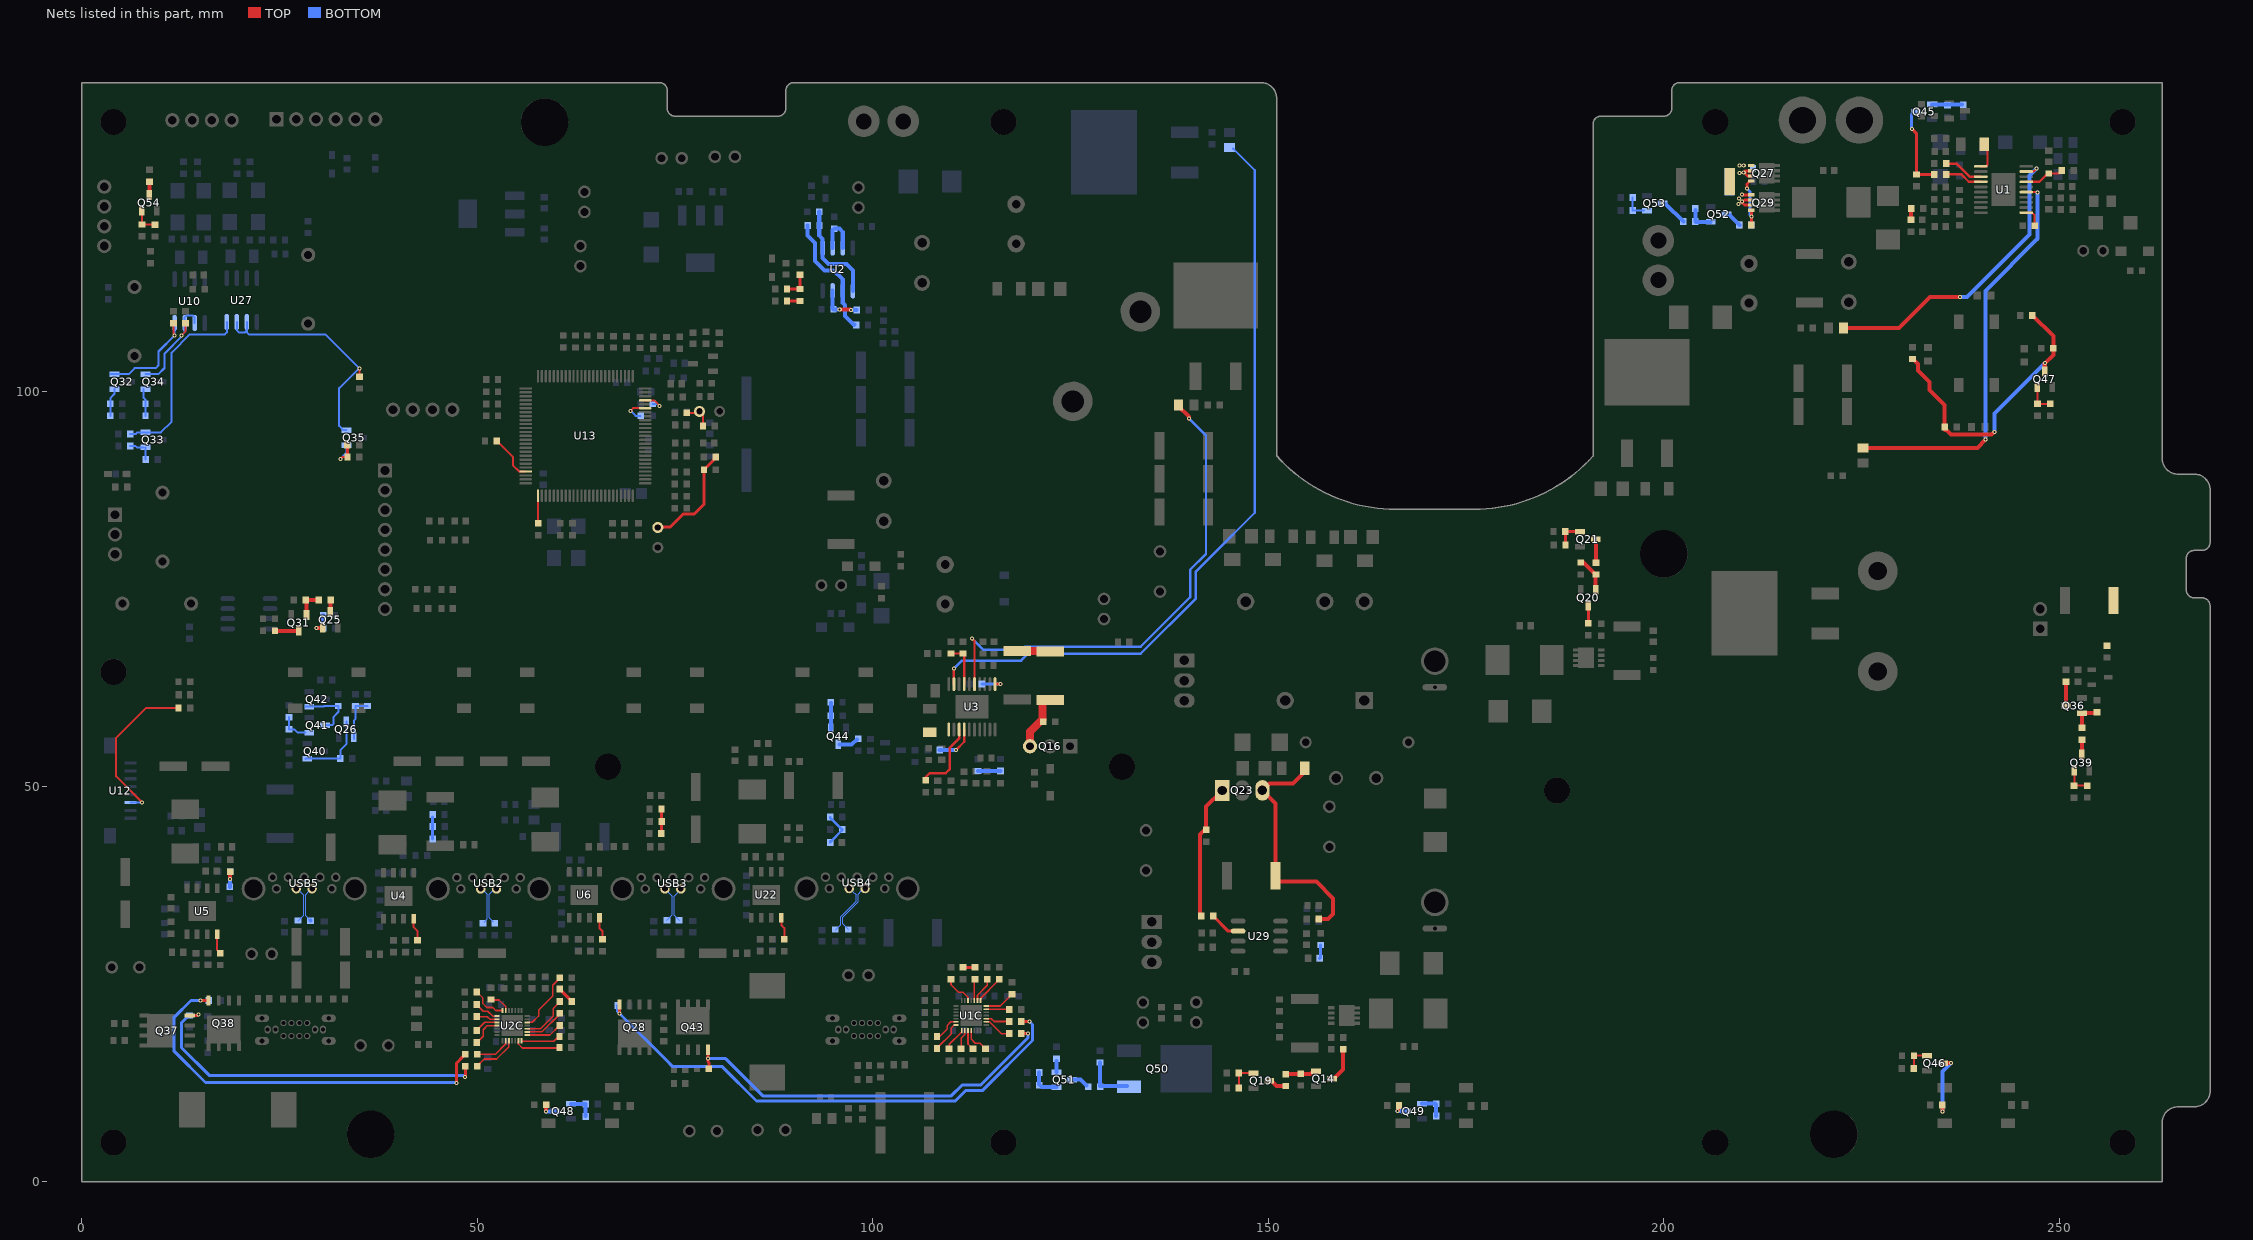
[diagram p0: the nets of this part, all layers, seen from the top]
# Altium PCB MISC84402.PcbDoc (part 8 of 12)
Units mm, origin at the board's own origin, x right, y up, seen from the top; angles counter-clockwise.
Board outline 269.06 x 139 mm, 4 copper layers (TOP, GND02, PWR03, BOTTOM), stack 0.732 mm thick; 694 components, 428 nets, 1859 pads, 1384 vias.

## Via types
v1: diameter 0.508, hole 0.254, TOP to BOTTOM, tented both sides, 1015 vias
v2: diameter 0.508, hole 0.254, TOP to BOTTOM, 243 vias
v3: diameter 0.508, hole 0.305, TOP to BOTTOM, 60 vias
v4: diameter 0.61, hole 0.305, TOP to BOTTOM, 55 vias
v5: diameter 0.61, hole 0.305, TOP to BOTTOM, tented both sides, 8 vias
v6: diameter 0.762, hole 0.381, TOP to BOTTOM, 2 vias
v7: diameter 0.762, hole 0.381, TOP to BOTTOM, tented both sides, 1 vias

## Nets (pads, with @x,y where several pads share a name; then routed paths per layer and width w, separated by ;. In a path a pad name is that pad's centre, name@x,y a point inside that pad or via, vN(x,y) a via of type N, cw(c..) or ccw(c..) an arc to the next point about the centre after c; other vN are vias at no path point) (continued)
NetQ14_1: Q14.1 R23.2 R29.1 | length 3.5
  TOP w0.508: R29.1@152.232,13.673 155.329,13.673 Q14.1@155.626,13.97
NetQ14_3: Q14.3 R61.1 | length 4.1
  TOP w0.508: Q14.3@158.032,13.047 158.233,13.047 159.436,14.249 R61.1@159.436,16.459
NetQ16_3: Q16.3 R50.1 R148.1 | length 5.5
  TOP w1.016: Q16.3@119.888,55.499 119.888,56.947 121.437,58.496 R50.1@121.437,60.342
NetQ19_1: Q19.1 R32.2 R65.1 | length 3.6
  TOP w0.254: R32.2@146.184,13.76 Q19.1@148.114,13.76 ; R65.1@146.294,11.887 R32.2@146.294,13.528
NetQ19_3: Q19.3 R29.2 | length 2.2
  TOP w0.508: Q19.3@150.114,12.81 150.334,12.81 151.003,12.141 R29.2@152.044,12.141
NETQ20_1: Q20.1 R35.2 R39.1 | length 4.2
  TOP w0.508: R35.2@189.789,78.384 191.385,76.788 Q20.1@191.385,74.879
NetQ20_3: Q20.3 R66.1 | length 2
  TOP w0.381: R66.1@190.444,70.619 Q20.3@190.444,72.599
NetQ21_1: Q21.1 R40.2 R44.1 | length 3.3
  TOP w0.381: R40.2@187.554,80.645 187.554,82.079 187.687,82.213 Q21.1@189.389,82.213
NetQ21_3: Q21.3 R39.2 | length 2.8
  TOP w0.508: R39.2@191.415,78.366 Q21.3@191.415,81.127
NETQ23_1: Q23.1 R240.2 R265.2 | length 17.4
  TOP w0.508: R240.2@141.63,33.706 141.326,34.01 141.326,43.917 R265.2@141.942,44.533 ; Q23.1@144.171,49.495 142.139,47.463 R265.2@142.139,44.533 ; R265.2@141.942,44.533 R265.2@142.139,44.533 ; R265.2@141.942,44.533 R265.2@142.139,44.533
NETQ23_3: Q23.3 R258.1 R316.2 R361.1 | length 31.1
  TOP w0.508: R361.1@154.432,51.689 153.111,50.368 150.114,50.368 Q23.3@149.251,49.505 150.902,47.854 150.902,43.272 R316.2@150.902,38.7 150.902,37.549 151.326,37.973 156.066,37.973 158.174,35.865 158.174,33.884 157.529,33.239 R258.1@156.354,33.239
NetQ25_1: Q25.1 R186.2 R193.1 | length 3.2
  TOP w0.508: v2(29.676,70.062) 29.686,70.053 Q25.1@30.455,70.053
  BOTTOM w0.508: v2(29.676,70.062) 30.489,70.062 R193.1@30.489,71.644
NetQ25_3: Q25.3 R100.1 | length 1.6
  TOP w0.508: Q25.3@31.41,72.069 R100.1@31.41,73.625
NETQ26_1: Q26.1 R95.2 R140.2 | length 5.8
  BOTTOM w0.254: Q26.1@34.377,55.992 Q26.1@34.377,56.242 34.377,58.319 34.57,58.512 R140.2@34.57,60.171 R95.2@36.094,60.171
NETQ26_3: Q26.3 Q40.1 R144.1 | length 9.5
  BOTTOM w0.254: Q40.1@28.24,53.498 28.301,53.559 28.49,53.559 R144.1@32.674,53.559 32.674,54.602 33.427,55.355 Q26.3@33.427,58.242
NETQ27_1: Q27.1 Q27.2 Q27.3 Q29.1 Q29.2 Q29.3 R26.2 R45.2 R67.1 | length 6
  TOP w0.381: v1(209.866,124.851) 209.907,124.81 Q29.1@211.06,124.81 ; v1(210.101,127.645) v1@210.12,127.645 ; Q29.3@211.06,123.51 210.191,123.51 209.866,123.835 210.191,124.16 Q29.2@211.06,124.16 ; Q27.3@211.06,127.193 210.572,127.193 v1@210.12,127.645 ; Q27.2@211.06,127.843 210.318,127.843 v1@210.12,127.645
  other v1: 209.892,123.937 210.101,128.534
  other v2: 209.448,123.647 209.499,124.358 209.575,127.584 209.575,128.524
NETQ27_4: Q27.4 Q29.4 R56.2 R60.2 | length 7.6
  TOP w0.381: v1(210.501,125.613) 210.501,126.162 210.882,126.543 Q27.4@211.06,126.543 ; Q29.4@211.06,122.699 Q29.4@211.06,122.86 ; R56.2@211.065,120.98 Q29.4@211.065,122.699
  BOTTOM w0.381: v1(210.501,125.613) 210.882,125.232 210.882,122.264 ; R60.2@211.055,120.99 v1@211.055,121.977
  other v1: 211.087,122.06
NETQ28_4: Q28.4 R126.1 R129.2 | length 66.1
  TOP w0.381: v1(67.971,21.301) Q28.4@67.971,22.431 ; R129.2@118.745,20.285 v1(119.787,20.285)
  BOTTOM w0.381: R126.1@67.726,22.317 67.726,21.546 v1(67.971,21.301) 73.897,15.375 ; 74.087,15.185 73.897,15.375 ; v1(119.787,20.285) v1@119.82,20.252 ; v1@119.837,20.269 120.193,19.914 120.193,17.882 113.894,11.582 111.76,11.582 110.429,10.252 85.278,10.252 80.899,14.63 74.641,14.63 73.897,15.375
NetQ31_1: Q31.1 R98.2 R100.2 | length 3.3
  TOP w0.508: Q31.1@28.39,71.697 R98.2@28.39,73.526 ; R98.2@28.473,73.558 R100.2@29.955,73.558
NetQ31_3: Q31.3 R42.1 | length 3
  TOP w0.508: R42.1@24.401,69.688 Q31.3@27.442,69.688
NETQ32_1: Q32.1 R91.2 R159.2 | length 3.6
  BOTTOM w0.254: R159.2@3.599,96.866 3.582,96.883 3.582,98.39 3.582,99.111 4.096,99.626 Q32.1@4.096,100.234
NETQ32_2: Q32.2 R154.1 U10.4 | length 14.3
  TOP w0.254: R154.1@11.583,108.567 11.583,107.28 11.71,107.153 v1(11.71,107.026)
  BOTTOM w0.254: Q32.2@3.614,102.134 Q32.2@4.096,102.134 5.911,102.134 6.664,102.887 9.331,102.887 9.678,103.234 9.678,104.994 v1(11.71,107.026) U10.4@11.71,108.603
NETQ33_1: Q33.1 R105.2 R165.2 | length 3.3
  BOTTOM w0.254: R105.2@6.104,93.073 R105.2@6.122,93.056 6.757,93.056 6.945,92.868 Q33.1@7.793,92.868 ; Q33.1@8.043,92.868 8.043,91.348 R165.2@8.061,91.33
NETQ33_2: Q33.2 R152.1 U27.4 | length 24
  BOTTOM w0.254: R152.1@6.104,94.58 6.811,94.58 6.999,94.768 Q33.2@8.043,94.768 9.975,94.768 11.329,96.122 11.329,104.858 13.624,107.153 18.06,107.153 18.314,107.407 U27.4@18.314,108.73
NETQ34_1: Q34.1 R93.2 R184.2 | length 3.5
  BOTTOM w0.254: Q34.1@7.809,100.234 7.809,99.124 8.036,98.898 R93.2@8.036,98.39 R184.2@8.036,96.866
NETQ34_2: Q34.2 R156.1 U10.2 U10.3 | length 14.1
  TOP w0.254: v1(12.599,107.026) 13.107,107.534 R156.1@13.107,108.567
  BOTTOM w0.254: Q34.2@8.059,102.134 9.667,102.134 10.44,102.907 10.44,104.74 12.599,106.899 v1(12.599,107.026) 12.98,107.407 U10.3@12.98,108.603 12.98,109.312 13.234,109.566 13.996,109.566 14.25,109.312 U10.2@14.25,108.603
NETQ35_1: Q35.1 R146.2 R176.2 | length 4.6
  TOP w0.254: v1(32.67,91.41) 32.919,91.659 R176.2@33.571,91.659
  TOP w0.381: R146.2@33.554,93.183 33.554,91.676 R176.2@33.571,91.659
  BOTTOM w0.254: v1(32.67,91.41) 33.433,92.173 Q35.1@33.433,93.157
NETQ35_2: Q35.2 R157.1 U27.2 U27.3 | length 30.6
  TOP w0.254: R157.1@35.078,101.819 v1(35.078,102.835)
  BOTTOM w0.254: U27.3@19.584,108.73 19.584,107.661 19.838,107.407 20.6,107.407 20.854,107.661 ; U27.2@20.854,108.73 20.854,107.661 ; Q35.2@33.433,95.057 33.061,95.057 32.512,95.606 32.512,100.355 v1@34.976,102.819 ; v1@35.019,102.776 v1(35.078,102.835) ; v1@35.047,102.865 v1(35.078,102.835) ; v1@35.052,102.87 30.769,107.153 21.108,107.153 20.854,107.407 20.854,107.661 ; v1@35.078,102.962 v1(35.078,102.835)
NetQ36_1: Q36.1 R288.2 R289.2 | length 3.5
  TOP w0.508: R288.2@252.85,57.487 Q36.1@252.85,59.29 R289.2@254.552,59.29
NetQ36_3: Q36.3 R71.1 | length 2.7
  TOP w0.508: Q36.3@250.85,60.24 R71.1@250.85,62.966
NETQ37_4: Q37.4 R201.2 R212.1 | length 45.6
  TOP w0.381: Q37.4@13.615,21.047 14.631,21.047 v1(14.758,21.174) ; v1(48.447,13.301) 48.464,13.319 R201.2@48.464,14.622
  BOTTOM w0.381: v1(14.758,21.174) 14.631,21.046 13.503,21.046 12.599,20.143 12.599,16.983 16.145,13.437 48.31,13.437 v1@48.447,13.3
NETQ38_4: Q38.4 R202.2 R209.1 | length 51.9
  TOP w0.381: v1(15.012,22.952) 15.025,22.939 Q38.4@16.028,22.939 ; v1(47.355,12.539) 47.355,15.021 R202.2@48.285,15.951 ; R202.2@48.285,16.146 R202.2@48.456,16.146
  BOTTOM w0.381: R209.1@16.037,22.952 v1(15.012,22.952) 13.782,22.952 11.659,20.828 11.659,16.526 15.612,12.573 47.319,12.573 v1@47.355,12.538
NetQ39_1: Q39.1 R272.1 R287.2 | length 3.3
  TOP w0.254: Q39.1@251.899,52.026 251.899,50.158 251.943,50.114 R272.1@253.289,50.114
NetQ39_3: Q39.3 R288.1 | length 1.7
  TOP w0.508: Q39.3@252.849,54.026 R288.1@252.849,55.736
NETQ41_1: Q41.1 R180.2 R188.1 | length 3.8
  BOTTOM w0.254: R180.2@26.188,58.774 R188.1@26.188,57.233 26.832,57.233 27.265,56.8 Q41.1@28.24,56.8
NETQ41_3: Q41.3 Q42.1 R319.1 | length 7.8
  BOTTOM w0.254: Q42.1@28.24,60.102 Q42.1@28.74,60.102 30.563,60.102 30.633,60.172 R319.1@32.411,60.171 32.411,59.419 31.81,58.818 31.81,57.929 31.631,57.75 Q41.3@30.74,57.75
NETQ43_4: Q43.4 R130.2 R131.1 | length 49.3
  TOP w0.381: Q43.4@79.147,16.728 v1(79.147,15.586) 79.147,15.205 79.265,15.087 R131.1@79.265,14.316 ; R130.2@118.745,18.761 v1(119.596,18.761)
  BOTTOM w0.381: v1(79.147,15.586) 81.392,15.586 86.091,10.887 109.896,10.887 111.252,12.243 113.614,12.243 119.583,18.212 v1@119.583,18.644 ; v1@119.596,18.644 v1(119.596,18.761)
NetQ44_1: Q44.1 R53.1 R73.2 | length 3.3
  BOTTOM w0.508: Q44.1@94.698,57.27 R73.2@94.698,60.535
NetQ44_3: Q44.3 R104.1 | length 2.5
  BOTTOM w0.508: Q44.3@95.775,55.287 97.324,55.287 R104.1@97.993,55.956
NetQ45_1: Q45.1 R308.2 R314.2 | length 3.8
  BOTTOM w0.508: Q45.1@233.902,136.239 R308.2@237.712,136.239
NetQ45_3: Q45.3 R52.1 R296.2 | length 10.4
  TOP w0.381: v2(231.394,133.121) 231.927,132.588 R296.2@231.927,127.372 ; R296.2@232.181,127.381 R52.1@234.197,127.381
  BOTTOM w0.381: v2(231.394,133.121) 231.292,133.223 231.292,134.925 Q45.3@231.673,135.306
NetQ46_1: Q46.1 R323.1 R325.2 | length 3.1
  TOP w0.254: R325.2@231.622,14.452 R323.1@231.622,15.96 Q46.1@233.232,15.96
NetQ46_3: Q46.3 R64.2 | length 9
  TOP w0.508: v2(235.204,8.915) R64.2@235.204,9.601 ; Q46.3@235.28,15.02 v2(236.313,15.02)
  BOTTOM w0.508: v2(235.204,8.915) 235.204,11.049 ; 235.204,10.279 235.204,11.049 ; v2@236.22,14.961 235.204,13.945 235.204,11.049
NetQ47_1: Q47.1 R332.1 R333.2 | length 3.8
  TOP w0.254: Q47.1@247.244,100.533 247.244,98.382 247.244,98.374 R332.1@248.86,98.374
NetQ47_3: Q47.3 R78.2 R79.2 R118.2 R187.2 | length 37.5
  TOP w0.508: R79.2@231.521,104.038 232.156,103.403 232.156,102.616 233.604,101.168 233.604,100.136 235.509,98.231 R118.2@235.509,95.453 ; R118.2@235.458,95.326 R118.2@235.518,95.267 ; R118.2@235.518,95.063 R118.2@235.518,95.267 ; R118.2@235.518,95.453 R118.2@235.518,95.267 ; v2@241.783,94.818 241.452,94.488 236.296,94.488 R118.2@235.518,95.267 ; R187.2@246.558,109.626 249.25,106.934 249.25,104.572 248.158,103.48 Q47.3@248.158,102.565 ; Q47.3@248.175,102.489 Q47.3@248.175,102.565
  BOTTOM w0.508: v2(241.783,94.844) 241.783,97.13 v2(248.183,103.53)
NetQ48_1: Q48.1 R334.1 R335.2 | length 3.3
  BOTTOM w0.508: Q48.1@61.842,9.874 63.646,9.874 63.646,8.363 R335.2@63.652,8.357
NetQ48_3: Q48.3 R194.2 | length 2
  TOP w0.508: v2@58.691,8.95 R194.2@58.691,9.754
  BOTTOM w0.508: v2(58.691,8.924) Q48.3@59.842,8.924
NetQ49_1: Q49.1 R336.1 R337.2 | length 3.3
  BOTTOM w0.508: Q49.1@169.411,9.899 171.088,9.899 171.196,9.791 R336.1@171.196,8.331
NetQ49_3: Q49.3 R195.2 | length 1.9
  TOP w0.508: v2@166.362,9.009 R195.2@166.362,9.838
  BOTTOM w0.508: v2(166.328,8.949) Q49.3@167.411,8.949
NetQ50_1: Q50.1 R348.2 R351.2 | length 6.4
  BOTTOM w0.508: R351.2@128.711,15.105 128.711,12.125 Q50.1@132.096,12.125
NetQ51_1: Q51.1 R349.1 R350.2 | length 3.7
  BOTTOM w0.508: R350.2@121.031,12.369 R349.1@121.031,13.859 ; R350.2@121.082,12.268 121.354,11.996 Q51.1@123.197,11.996
NetQ51_2: Q51.2 R338.2 | length 1.4
  BOTTOM w0.508: Q51.2@123.197,13.896 R338.2@123.197,15.284
NetQ51_3: Q51.3 R348.1 | length 2.1
  BOTTOM w0.508: Q51.3@125.197,12.946 126.272,12.946 R348.1@127.025,12.192
NetQ52_1: Q52.1 R352.2 R353.2 | length 3.4
  BOTTOM w0.508: R353.2@204.013,122.86 204.013,121.437 204.057,121.393 Q52.1@205.925,121.393
NetQ52_3: Q52.3 R60.1 | length 1.8
  BOTTOM w0.508: Q52.3@208.305,122.233 R60.1@209.548,120.99
NetQ53_1: Q53.1 R177.1 R191.2 | length 2.9
  BOTTOM w0.254: R191.2@196.048,122.834 Q53.1@197.485,122.834 ; R191.2@196.06,123.035 R177.1@196.06,124.45
NetQ53_3: Q53.3 R352.1 | length 3.2
  BOTTOM w0.508: Q53.3@200.212,123.673 R352.1@202.464,121.421
NetQ54_1: Q54.1 R364.2 R365.1 | length 3
  TOP w0.254: Q54.1@7.603,122.42 7.603,121.039 R364.2@9.229,121.039
NetQ54_3: Q54.3 R363.2 | length 1.8
  TOP w0.508: Q54.3@8.526,124.79 R363.2@8.526,126.602
NetR1_1: R1.1 U1.1 | length 3.7
  TOP w0.305: U1.1@240.078,128.401 240.695,128.401 240.919,128.625 240.919,130.765 R1.1@240.493,131.191
NETR2_1: R2.1 R15.2 U3.17 | length 5.5
  TOP w0.305: R15.2@109.855,66.811 R2.1@111.379,66.811 111.547,66.643 U3.17@111.547,62.944
NETR7_1: R7.1 R210.2 | length 2.8
  BOTTOM w0.508: R7.1@113.284,51.961 R210.2@116.111,51.961
NETR10_2: R10.2 U1.3 | length 5.1
  TOP w0.305: R10.2@235.703,128.749 237.011,128.749 238.659,127.101 U1.3@240.078,127.101
NETR11_2: R11.2 U3.3 | length 9.3
  TOP w0.305: R11.2@106.68,50.791 106.68,51.181 107.188,51.689 109.22,51.689 109.728,52.197 109.728,54.913 110.897,56.082 U3.3@110.897,57.198
NetR13_1: R13.1 R50.2 | length 2.9
  TOP w1.016: R13.1@118.238,67.115 R50.2@121.15,67.115
NetR17_1: R17.1 R24.2 R76.2 | length 2.8
  BOTTOM w0.381: R76.2@44.34,43.342 R17.1@44.34,46.144
NETR21_1: R21.1 U1.11 | length 2.5
  TOP w0.254: U1.11@245.824,122.551 246.544,122.551 246.879,122.216 R21.1@246.879,120.904
NetR30_2: R30.2 R63.2 R103.1 | length 2.8
  TOP w0.508: v1(18.695,38.319) R103.1@18.695,39.141
  BOTTOM w0.508: R30.2@18.695,37.302 v1(18.695,38.319) ; v1@18.694,38.354 18.694,39.203 R63.2@18.745,39.253
NETR33_1: R33.1 R57.2 R256.1 | length 13.7
  TOP w0.254: R256.1@80.154,91.659 R256.1@80.154,91.786
  TOP w0.305: R256.1@79.883,91.289 R256.1@79.883,91.364
  TOP w0.381: R57.2@72.873,82.779 74.346,82.779 75.999,84.432 77.396,84.432 78.647,85.683 R33.1@78.647,90.053 80.137,91.543 R256.1@80.137,91.567
NETR34_1: R34.1 R136.1 | length 1.4
  TOP w0.305: R34.1@231.267,123.054 R34.1@231.276,123.063
  TOP w0.508: R136.1@231.267,121.657 R34.1@231.267,123.054
NetR37_2: R37.2 U3.4 | length 5.1
  TOP w0.305: v1(110.49,54.61) 111.547,55.667 U3.4@111.547,57.198
  BOTTOM w0.508: R37.2@108.449,54.61 v1(110.49,54.61)
NETR43_1: R43.1 U3.11 | length 3
  TOP w0.381: U3.11@115.498,62.944 v2(116.151,62.944) v2@116.202,62.944
  BOTTOM w0.381: R43.1@113.774,62.941 v2@116.078,62.941
NETR46_1: R46.1 R163.1 R257.1 | length 3.7
  TOP w0.254: R257.1@76.471,97.247 78.521,97.247 R46.1@78.521,95.596
NetR52_2: R52.2 U1.4 | length 5
  TOP w0.305: R52.2@235.703,127.381 237.236,127.381 ; 236.982,127.381 237.236,127.381 ; U1.4@240.078,126.451 238.547,126.451 237.617,127.381 237.236,127.381
NetR54_1: R54.1 U3.1
NETR55_2: R55.2 R274.1 U1.17 | length 5.1
  TOP w0.305: U1.17@245.824,126.451 247.482,126.451 248.53,127.499 R274.1@248.666,127.499 249.927,127.499 R55.2@250.317,127.889
  TOP w0.381: R274.1@248.666,127.499 R274.1@248.675,127.508
NetR58_2: R58.2 R62.1 R87.2 | length 3
  TOP w0.381: R87.2@73.296,44.034 73.296,44.086 R58.2@73.296,45.558 R62.1@73.296,47.082
NetR74_2: R74.2 U3.19 | length 97.3
  TOP w0.305: v1(110.236,64.897) 110.247,64.886 U3.19@110.247,62.944
  BOTTOM w0.305: v1(110.236,64.897) 111.252,65.913 118.745,65.913 119.634,66.802 133.87,66.802 140.843,73.775 140.843,77.165 142.875,79.197 148.285,84.607 148.285,127.914 R74.2@145.567,130.632
NETR75_1: R75.1 R294.2 | length 1.7
  TOP w0.381: R75.1@89.145,111.379 90.796,111.379 R294.2@90.805,111.388
NETR80_2: R80.2 U13.20 | length 3.5
  TOP w0.254: v1(69.368,97.501) 69.693,97.826 U13.20@71.203,97.826
  BOTTOM w0.254: v1(69.368,97.501) 70.003,96.866 R80.2@70.647,96.866
NetR84_2: R84.2 USB3.2 | length 4.1
  BOTTOM w0.127: R84.2@73.965,33.087 74.651,33.773 74.651,36.144 USB3.2@74.092,36.703
NetR85_2: R85.2 R96.2 R99.1 | length 4.6
  BOTTOM w0.305: R85.2@94.624,42.926 R85.2@94.624,43.053 ; R99.1@94.624,45.974 R99.1@94.624,46.101 ; R99.1@94.64,45.898 R99.1@94.742,45.898 ; R99.1@94.666,45.974 R99.1@94.742,45.898 ; R85.2@94.691,43.053 96.105,44.467 R96.2@96.105,44.552 94.759,45.898 R99.1@94.742,45.898 ; R96.2@96.037,44.425 R96.2@96.037,44.552 ; R96.2@96.13,44.552 R96.2@96.13,44.577
NetR90_2: R90.2 USB3.3 | length 4.2
  BOTTOM w0.127: R90.2@75.489,33.096 75.489,33.122 74.905,33.706 74.905,36.144 USB3.3@75.565,36.805
NetR92_2: R92.2 USB5.3 | length 4.3
  BOTTOM w0.127: 28.27,36.22 28.27,36.144 ; USB5.3@28.753,36.805 28.27,36.322 28.27,36.144 ; R92.2@28.88,33.045 28.27,33.655 28.27,36.144
  BOTTOM w0.508: R92.2@28.88,33.045 R92.2@28.905,33.045
NetR97_2: R97.2 USB5.2 | length 4.4
  BOTTOM w0.127: R97.2@27.331,33.054 28.016,33.739 28.016,36.271 USB5.2@27.381,36.906
NetR101_2: R101.2 U3.15 | length 63.5
  TOP w0.305: v1(112.522,68.707) 112.847,68.382 U3.15@112.847,62.944
  TOP w0.508: R101.2@138.649,97.901 R101.2@138.649,98.053 ; R101.2@138.649,98.222 R101.2@138.649,98.053 ; v1@139.954,96.545 139.954,96.749 R101.2@138.649,98.053
  BOTTOM w0.305: v1@112.53,68.699 113.919,67.31 118.88,67.31 119.253,67.683 133.862,67.683 140.132,73.953 140.132,77.419 142.113,79.4 142.113,94.361 v1(139.954,96.52)
NetR102_2: R102.2 USB2.3 | length 4.5
  BOTTOM w0.127: R102.2@51.994,32.893 51.511,33.376 51.511,36.347 USB2.3@52.095,36.932
NetR107_2: R107.2 R294.1 R295.2 | length 3.5
  TOP w0.381: R295.2@89.145,112.903 90.796,112.903 R294.1@90.805,112.894 R107.2@90.805,114.69
NetR112_2: R112.2 R142.1 U2.2 | length 15.7
  BOTTOM w0.508: R142.1@91.746,120.947 91.746,119.658 92.659,118.745 92.659,116.434 93.853,115.24 95.047,115.24 96.19,114.097 96.19,111.15 96.495,110.846 96.495,109.474 R112.2@97.612,108.356 ; R112.2@97.65,108.394 R112.2@97.663,108.382
NetR120_2: R120.2 USB2.2 | length 4.4
  BOTTOM w0.127: USB2.2@50.749,36.855 51.257,36.347 51.257,33.249 R120.2@50.851,32.842
NetR121_2: R121.2 U1.19 | length 38.6
  TOP w0.305: U1.19@245.824,127.751 246.75,127.751 v1(247.142,128.143)
  TOP w0.508: R121.2@222.742,107.95 229.743,107.95 233.68,111.887 v1(237.465,111.887)
  BOTTOM w0.508: v1@237.439,111.887 v1(237.465,111.887) 238.354,111.887 246.253,119.786 246.253,127.254 v1(247.142,128.143)
NetR122_1: R122.1 R189.2 | length 2.1
  TOP w0.381: R122.1@60.403,24.401 60.403,24.365 R189.2@61.849,22.919 ; R189.2@61.849,22.911 R189.2@61.849,22.919 ; R189.2@61.891,22.877 R189.2@61.849,22.919
NetR123_2: R123.2 USB4.3 | length 6.2
  BOTTOM w0.127: R123.2@96.891,31.928 96.876,31.928 96.164,32.639 96.164,33.452 98.12,35.408 98.12,36.398 USB4.3@98.552,36.83
NetR124_2: R124.2 R368.1
NetR125_2: R125.2 U1.15 | length 51.3
  TOP w0.254: U1.15@245.824,125.151 v1@247.213,125.151
  TOP w0.508: R125.2@225.171,92.821 239.633,92.821 v1(240.665,93.853)
  BOTTOM w0.508: v1(240.665,93.853) 240.665,98.273 240.665,112.649 247.269,119.253 v1(247.269,125.095)
NETR127_1: R127.1 U1C.21 | length 3.9
  TOP w0.203: U1C.21@114.328,22.247 116.091,22.247 R127.1@117.602,23.758
NETR128_1: R128.1 U1C.20 | length 2.9
  TOP w0.203: U1C.20@114.328,21.847 R128.1@117.193,21.847 ; R128.1@117.193,21.809 R128.1@117.238,21.809
NETR129_1: R129.1 U1C.17 | length 3.1
  TOP w0.203: U1C.17@114.328,20.647 114.98,20.647 115.342,20.285 R129.1@117.238,20.285
NETR130_1: R130.1 U1C.16 | length 3.5
  TOP w0.203: U1C.16@114.328,20.247 114.745,20.247 116.231,18.761 R130.1@117.238,18.761
NetR132_2: R132.2 U5.8 | length 2.6
  TOP w0.254: U5.8@17.098,31.346 17.098,29.314 R132.2@17.479,28.933
NetR133_2: R133.2 U4.8 | length 2.9
  TOP w0.254: U4.8@41.936,33.251 41.936,32.223 42.444,31.715 R133.2@42.444,30.571
NetR135_2: R135.2 U6.8 | length 2.8
  TOP w0.254: U6.8@65.431,33.378 65.431,32.096 65.812,31.715 R135.2@65.812,30.698
NetR137_2: R137.2 USB4.2 | length 6.2
  BOTTOM w0.127: R137.2@95.25,31.919 95.292,31.919 95.91,32.537 95.91,33.557 97.866,35.513 97.866,36.297 USB4.2@97.384,36.779
NetR142_2: R142.2 R271.1 U2.1 U2.5 | length 13.1
  BOTTOM w0.508: R271.1@93.218,122.666 93.218,120.734 93.218,119.634 93.649,119.203 U2.5@93.649,118.087 93.649,116.79 94.361,116.078 96.647,116.078 97.459,115.266 U2.1@97.459,112.677
NetR145_2: R145.2 R290.2 U2.3 | length 5.1
  TOP w0.508: v2(95.809,110.338) 97.104,110.338 v2(97.206,110.236)
  BOTTOM w0.508: R145.2@94.919,110.516 U2.3@94.919,112.677 ; R145.2@95.013,110.338 v2(95.809,110.338) ; v2(97.206,110.236) R290.2@97.951,110.236
NetR147_1: R147.1 U2.6 U2.7 | length 5.8
  BOTTOM w0.508: U2.6@94.919,118.087 94.919,120.328 R147.1@95.123,120.532 95.775,120.532 96.189,120.117 U2.7@96.189,118.087
NETR149_1: R149.1 R155.2 | length 1.7
  BOTTOM w0.381: R155.2@156.481,28.286 156.617,28.422 R149.1@156.617,29.954
NETR151_1: R151.1 U1C.24 | length 2.5
  TOP w0.203: U1C.24@112.821,22.954 112.821,25.445 R151.1@112.827,25.451
NETR151_2: R151.2 R196.1 | length 1.5
  TOP w0.381: R196.1@111.405,27.125 R151.2@112.929,27.125
NETR161_1: R161.1 U1C.23 | length 3.2
  TOP w0.203: U1C.23@113.221,22.954 113.221,23.625 114.453,24.857 R161.1@114.453,25.619
NETR162_1: R162.1 U1C.22 | length 3.4
  TOP w0.203: U1C.22@113.621,22.954 113.621,23.222 R162.1@115.824,25.425
NETR170_2: R170.2 U1C.6 | length 3.4
  TOP w0.203: R170.2@108.153,18.39 108.458,18.39 109.423,19.355 109.423,19.812 109.858,20.247 U1C.6@110.513,20.247
  TOP w0.254: R170.2@108.103,18.38 R170.2@108.153,18.38
NETR173_2: R173.2 U1C.7 | length 4.1
  TOP w0.203: R173.2@108.204,17.018 109.931,18.745 109.931,19.507 110.271,19.847 U1C.7@110.513,19.847
  TOP w0.254: R173.2@108.103,16.856 R173.2@108.234,16.988
NETR175_2: R175.2 U1C.8 | length 3
  TOP w0.203: R175.2@109.652,17.069 109.652,17.399 111.221,18.968 U1C.8@111.221,19.139
  TOP w0.254: R175.2@109.627,16.838 R175.2@109.627,17.069
NETR178_2: R178.2 U1C.9 | length 2.5
  TOP w0.203: R178.2@111.176,17.069 111.176,18.212 111.621,18.657 U1C.9@111.621,19.139
  TOP w0.254: R178.2@111.151,16.856 R178.2@111.151,17.069
NETR179_2: R179.2 U1C.10 | length 2.7
  TOP w0.203: 112.021,17.637 112.021,17.932 ; U1C.10@112.021,19.139 112.021,18.085 112.021,17.932 ; R179.2@112.446,17.018 112.021,17.443 112.021,17.932
  TOP w0.254: R179.2@112.675,16.847 R179.2@112.675,16.983
NetR181_1: R181.1 U1C.11 | length 3.1
  TOP w0.203: U1C.11@112.421,19.139 112.421,18.084 112.954,17.551 113.538,17.551 R181.1@114.021,17.069
NETR182_1: R182.1 U2C.22 | length 4.9
  TOP w0.203: U2C.22@56.598,18.577 U2C.22@56.289,18.577 59.166,18.577 R182.1@60.274,19.685
  TOP w0.254: R182.1@60.275,19.684 R182.1@60.395,19.804
NETR185_1: R185.1 U2C.23 | length 5.1
  TOP w0.203: U2C.23@56.289,18.977 58.169,18.977 R185.1@60.35,21.158
  TOP w0.254: R185.1@60.288,21.221 R185.1@60.395,21.328
NetR189_1: R189.1 U2C.24 | length 6.2
  TOP w0.203: U2C.24@56.289,19.377 57.985,19.377 59.588,20.98 59.588,21.92 R189.1@60.223,22.555
  TOP w0.254: R189.1@60.245,22.534 60.385,22.674 R189.1@60.385,22.877
NETR199_1: R199.1 U2C.21 | length 5.1
  TOP w0.203: U2C.21@55.582,17.805 U2C.21@55.582,17.869 ; U2C.21@55.601,17.805 55.626,17.78 59.639,17.78 R199.1@60.147,18.288
  TOP w0.254: R199.1@60.216,18.22 R199.1@60.377,18.381
NETR200_1: R200.1 U2C.20 | length 6
  TOP w0.203: U2C.20@55.182,17.729 U2C.20@55.182,17.869 55.182,17.437 55.677,16.942 R200.1@60.122,16.942
  TOP w0.254: R200.1@60.122,16.984 R200.1@60.377,16.984
NETR201_1: R201.1 U2C.17 | length 5.8
  TOP w0.203: R201.1@49.987,14.681 50.851,15.545 52.426,15.545 53.982,17.101 U2C.17@53.982,17.869
  TOP w0.381: R201.1@49.971,14.622 R201.1@49.987,14.622
NETR202_1: R202.1 U2C.16 | length 4.6
  TOP w0.203: R202.1@50.216,16.154 52.273,16.154 53.582,17.463 U2C.16@53.582,17.869
  TOP w0.381: R202.1@49.962,16.146 R202.1@50.216,16.146
NETR211_2: R211.2 U2C.6 | length 2.7
  TOP w0.203: R211.2@51.714,23.012 52.324,23.012 52.73,23.012 53.569,22.174 U2C.6@53.569,21.717 ; U2C.6@53.582,21.684 U2C.6@53.582,21.717
NETR213_2: R213.2 U2C.7 | length 4.4
  TOP w0.203: R213.2@50.114,23.876 R213.2@50.203,23.787 ; R213.2@50.19,23.774 50.698,23.266 50.698,22.555 51.194,22.06 51.93,22.06 52.306,21.684 U2C.7@53.182,21.684
NETR214_2: R214.2 U2C.8 | length 2.8
  TOP w0.203: R214.2@50.216,22.098 50.724,21.59 51.308,21.59 51.921,20.977 U2C.8@52.474,20.977
  TOP w0.254: R214.2@49.937,22.444 R214.2@49.987,22.444
NETR215_2: R215.2 U2C.9 | length 2.7
  TOP w0.203: R215.2@49.886,20.904 51.257,20.904 51.585,20.577 U2C.9@52.474,20.577
NETR216_2: R216.2 U2C.10 | length 2.7
  TOP w0.203: R216.2@50.114,19.38 50.911,20.177 U2C.10@52.474,20.177
NETR217_1: R217.1 U13.72 | length 5.9
  TOP w0.254: R217.1@52.468,93.691 54.483,91.676 54.483,90.613 55.271,89.826 U13.72@56.103,89.826
NetR218_1: R218.1 U2C.11 | length 3.7
  TOP w0.203: R218.1@50.114,17.805 50.724,18.415 50.724,19.253 51.247,19.777 U2C.11@52.474,19.777
NETR222_1: R222.1 U13.76 | length 3.5
  TOP w0.254: U13.76@57.653,86.776 57.653,83.29 R222.1@57.684,83.259
NETR237_2: R237.2 U13.22 | length 3.1
  TOP w0.254: U13.22@71.203,98.826 72.361,98.826 v1(73.051,98.136)
  BOTTOM w0.254: R237.2@72.153,98.39 72.797,98.39 v1(73.051,98.136)
NETR240_1: R240.1 U29.6 | length 3.9
  TOP w0.381: R240.1@143.019,33.62 144.924,31.715 U29.6@146.172,31.715
NetR292_2: R292.2 U22.8 | length 2.8
  TOP w0.254: U22.8@88.418,33.378 88.418,32.486 88.799,32.105 R292.2@88.799,30.69
NETR307_2: R307.2 U2C.26 | length 7.5
  TOP w0.203: U2C.26@56.289,20.177 56.93,20.177 57.734,20.98 57.734,21.717 59.538,23.52 59.538,24.867 R307.2@60.3,25.629
NETR309_2: R309.2 U1C.26 | length 3.9
  TOP w0.203: R309.2@109.881,25.636 109.881,24.933 110.846,23.968 111.414,23.968 112.021,23.361 U1C.26@112.021,22.954
NETR322_1: R322.1 U12.6 | length 20.4
  TOP w0.254: v2@7.58,47.992 v2(7.593,47.979) ; v2@7.595,48.006 4.331,51.27 4.331,56.147 8.128,59.944 R322.1@12.201,59.944
  BOTTOM w0.254: U12.6@6.126,47.979 v2(7.593,47.979)